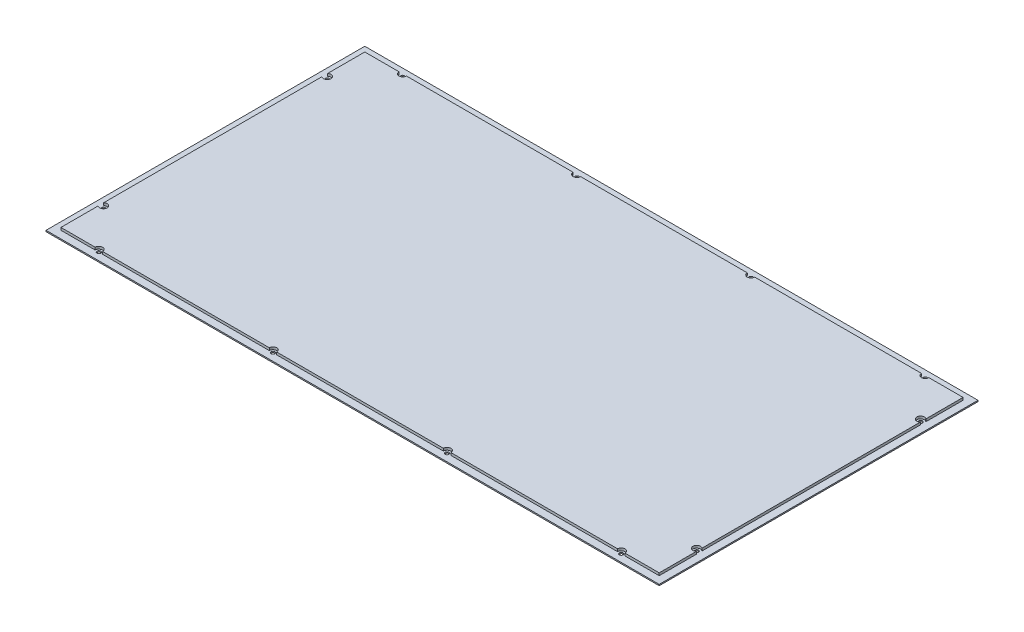
SolidWorks part; units mm, degrees
ref_plane "Front Plane" through (0, 0, 0) normal (0, 0, 1) x (1, 0, 0)
ref_plane "Top Plane" through (0, 0, 0) normal (0, 1, 0) x (1, 0, 0)
ref_plane "Right Plane" through (0, 0, 0) normal (1, 0, 0) x (0, 0, -1)
sketch "Sketch1" plane through (0, 0, 0) normal (0, 1, 0) x (1, 0, 0)
  line L1 (-246.5, 128.15) -> (246.5, 128.15)
  line L2 (-246.5, 128.15) -> (-246.5, -128.15)
  line L3 (-246.5, -128.15) -> (246.5, -128.15)
  line L4 (246.5, 128.15) -> (246.5, -128.15)
  line L5 (-246.5, 128.15) -> (246.5, -128.15) construction
  line L6 (-246.5, -128.15) -> (246.5, 128.15) construction
  point P0 (0, 0)
  dimension "D1" = 493
  dimension "D2" = 256.3
extrude "Boss-Extrude1" add sketch "Sketch1" along normal mid plane 3
sketch "Sketch2" plane through (0, 1.5, 0) normal (0, 1, 0) x (1, 0, 0)
  line L14 (240.5, -122.15) -> (240.5, 122.15)
  line L15 (-240.5, -122.15) -> (240.5, -122.15)
  line L16 (-240.5, 122.15) -> (-240.5, -122.15)
  line L17 (240.5, 122.15) -> (-240.5, 122.15)
  line L18 (240.5, -122.15) -> (240.5, 122.15)
  line L19 (-240.5, -122.15) -> (240.5, -122.15)
  line L20 (-240.5, 122.15) -> (-240.5, -122.15)
  line L21 (240.5, 122.15) -> (-240.5, 122.15)
  line L22 (246.5, -128.15) -> (246.5, 128.15)
  line L23 (246.5, 128.15) -> (-246.5, 128.15)
  line L24 (-246.5, 128.15) -> (-246.5, -128.15)
  line L25 (-246.5, -128.15) -> (246.5, -128.15)
  line L26 (246.5, -128.15) -> (246.5, 128.15)
  line L27 (246.5, 128.15) -> (-246.5, 128.15)
  line L28 (-246.5, 128.15) -> (-246.5, -128.15)
  line L29 (-246.5, -128.15) -> (246.5, -128.15)
  dimension "D1" = 6
  dimension "D2" = 0
extrude "Cut-Extrude1" cut sketch "Sketch2" against normal blind 2
sketch "Sketch3" plane through (0, 1.5, 0) normal (0, 1, 0) x (1, 0, 0)
  line L0 (0, 164.2174) -> (0, -184.3099) construction
  line L1 (240.5, 122.15) -> (-240.5, 122.15) construction
  circle A0 centre (-70, 122.15) radius 1.5
  circle A1 centre (-210, 122.15) radius 1.5
  circle A2 centre (70, 122.15) radius 1.5
  circle A3 centre (210, 122.15) radius 1.5
  dimension "D1" = 3
  dimension "D2" = 3
  dimension "D3" = 70
  dimension "D4" = 140
extrude "Cut-Extrude2" cut sketch "Sketch3" against normal through all
mirror "Mirror1" about plane through (0, 0, 0) normal (0, 0, 1) of "Cut-Extrude2"
sketch "Sketch4" plane through (0, 1.5, 0) normal (0, 1, 0) x (1, 0, 0)
  line L0 (-307.782, 0) -> (281.8939, 0) construction
  line L2 (-246.5, 128.15) -> (-246.5, -128.15) construction
  circle A0 centre (-238.5, 90) radius 1.5
  circle A1 centre (-238.5, -90) radius 1.5
  dimension "D1" = 3
  dimension "D2" = 90
  dimension "D3" = 8
extrude "Cut-Extrude3" cut sketch "Sketch4" against normal through all
mirror "Mirror2" about plane through (0, 0, 0) normal (1, 0, 0) of "Cut-Extrude3"
sketch "Sketch5" plane through (0, 1.5, 0) normal (0, 1, 0) x (1, 0, 0)
  circle A0 centre (-210, 122.15) radius 3
  circle A1 centre (-70, 122.15) radius 3
  circle A2 centre (70, 122.15) radius 3
  circle A3 centre (210, 122.15) radius 3
  circle A4 centre (238.5, 90) radius 3
  circle A5 centre (238.5, -90) radius 3
  circle A6 centre (210, -122.15) radius 3
  circle A7 centre (70, -122.15) radius 3
  circle A8 centre (-70, -122.15) radius 3
  circle A9 centre (-210, -122.15) radius 3
  circle A10 centre (-238.5, -90) radius 3
  circle A11 centre (-238.5, 90) radius 3
  dimension "D1" = 6
  dimension "D2" = 6
  dimension "D3" = 6
  dimension "D4" = 6
  dimension "D5" = 6
  dimension "D6" = 6
  dimension "D7" = 6
  dimension "D8" = 6
  dimension "D9" = 6
  dimension "D10" = 6
  dimension "D11" = 6
  dimension "D12" = 6
extrude "Cut-Extrude4" cut sketch "Sketch5" against normal up to surface (2 mm away) up to face at (0, -0.5, 0)
